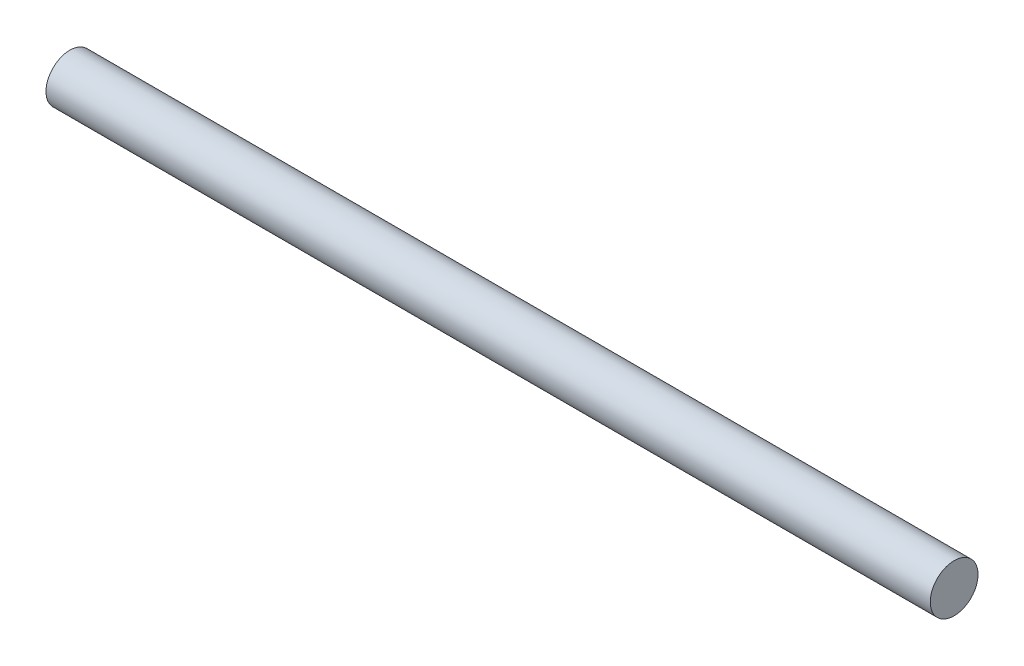
from build123d import *

# Parameters (mm, degrees)
SKETCH1_W = 185
SKETCH1_H = 10


with BuildPart() as part:
    # Sketch1 → Revolve1 (revolve)
    with BuildSketch(Plane.XY, mode=Mode.PRIVATE) as revolve1_sk:
        with Locations((-92.5, 5)):
            Rectangle(SKETCH1_W, SKETCH1_H)
    revolve1 = revolve(revolve1_sk.sketch.rotate(Axis((-202.604499093, 0, 0), (1, 0, 0)), 90), axis=Axis((-202.604499093, 0, 0), (1, 0, 0)))

    # Mirror1: Revolve1 across plane
    add(revolve1.mirror(Plane(origin=(0, 0, 0), x_dir=(0, 0, 1), z_dir=(1, 0, 0))))


solid = part.part
